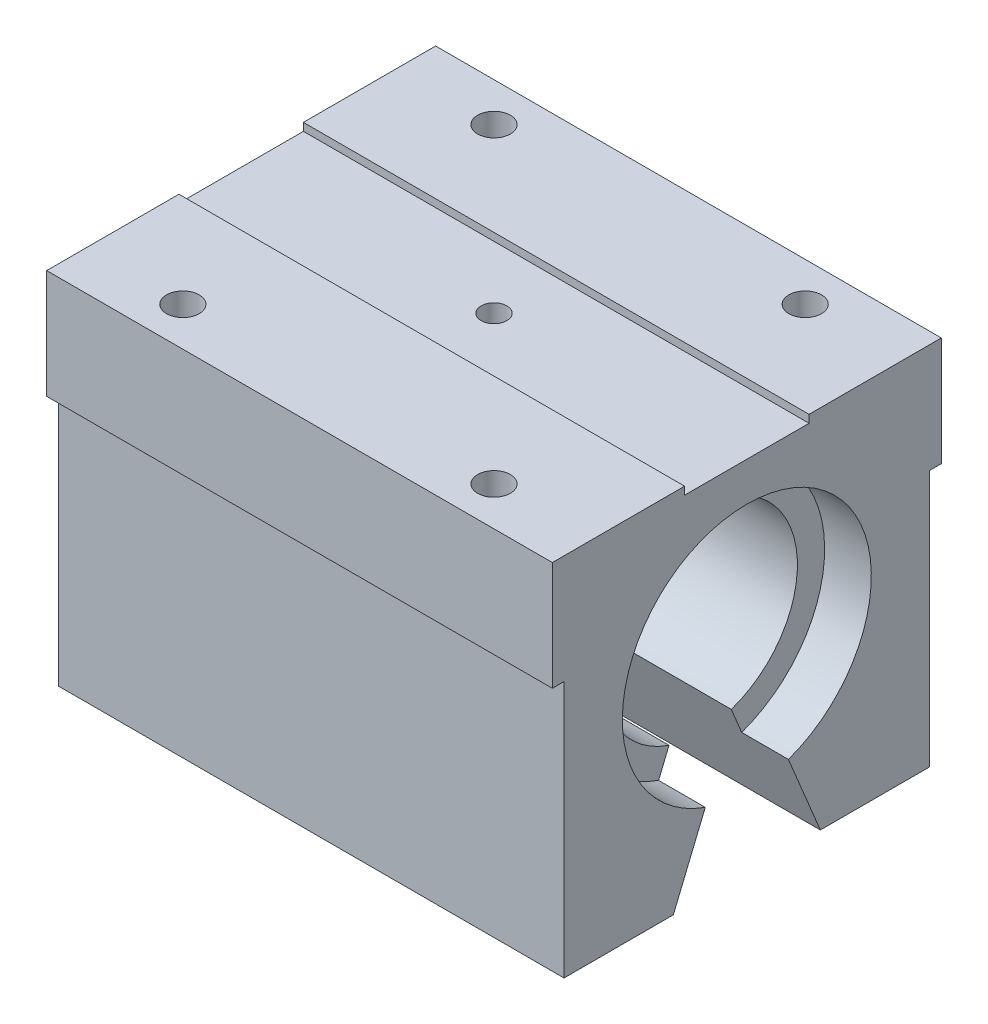
SolidWorks part; units mm, degrees
material "普通碳钢"
ref_plane "Front Plane" through (0, 0, 0) normal (0, 0, 1) x (1, 0, 0)
ref_plane "Top Plane" through (0, 0, 0) normal (0, 1, 0) x (1, 0, 0)
ref_plane "Right Plane" through (0, 0, 0) normal (1, 0, 0) x (0, 0, -1)
sketch "Sketch1" plane through (0, 0, 0) normal (1, 0, 0) x (0, 0, -1)
  line L0 (0, 0) -> (0, 31.1806) construction
  line L4 (-23.5, -25) -> (-9.4499, -25)
  line L5 (-25, 8) -> (-25, 22)
  line L6 (-8, 22) -> (-8, 21)
  line L8 (-8, 21) -> (8, 21)
  line L9 (-25, 22) -> (-8, 22)
  line L10 (8, 22) -> (8, 21)
  line L11 (8, 22) -> (25, 22)
  line L12 (-23.5, -25) -> (-23.5, 8)
  line L13 (23.5, -25) -> (23.5, 8)
  line L14 (-25, 8) -> (-23.5, 8)
  line L15 (25, 8) -> (25, 22)
  line L16 (-9.4499, -25) -> (-4, -11.8427)
  line L17 (23.5, 8) -> (25, 8)
  line L18 (9.4499, -25) -> (23.5, -25)
  line L20 (9.4499, -25) -> (4, -11.8427)
  arc A0 (4, -11.8427) -> (-4, -11.8427) centre (0, 0) ccw
  dimension "D1" = 25
  dimension "D7" = 22
  dimension "D10" = 8
  dimension "D2" = 45
  dimension "D3" = 47
  dimension "D4" = 50
  dimension "D5" = 16
  dimension "D6" = 1
  dimension "D8" = 1.5
  dimension "D9" = 14
extrude "Extrude1" add sketch "Sketch1" along normal blind 65
sketch "Sketch2" plane through (65, 0, 0) normal (1, 0, 0) x (0, 0, -1)
  circle A0 centre (0, 0) radius 16
  dimension "D1" = 32
extrude "Extrude2" cut sketch "Sketch2" against normal blind 6
sketch "Sketch3" plane through (0, 0, 0) normal (-1, 0, 0) x (0, 0, 1)
  arc A0 (5.3417, -15.082) -> (-5.3417, -15.082) centre (0, 0) ccw construction
  circle A2 centre (0, 0) radius 16
extrude "Extrude3" cut sketch "Sketch3" against normal blind 6
sketch "Sketch4" plane through (0, 22, 0) normal (0, 1, 0) x (1, 0, 0)
  line L0 (32.5, 25) -> (32.5, 0) construction
  line L1 (65, 25) -> (0, 25) construction
  line L2 (0, 0) -> (55.8292, 0) construction
  line L3 (12.5, -20) -> (52.5, -20) construction
  line L4 (12.5, -20) -> (12.5, 20) construction
  line L5 (12.5, 20) -> (52.5, 20) construction
  line L6 (52.5, -20) -> (52.5, 20) construction
  dimension "D1" = 40
  dimension "D2" = 40
hole_wizard "M5x0.8 Tapped Hole1" positions "3DSketch1" profile "Sketch5" tap size "M5x0.8" standard "Ansi Metric"
sketch3d "3DSketch1"
  point P0 (12.5, 22, -20)
  point P3 (52.5, 22, -20)
  point P6 (12.5, 22, 20)
  point P9 (52.5, 22, 20)
sketch "Sketch5" plane through (12.5, 22, -20) normal (1, 0, 0) x (0, 0, 1)
  line L0 (0, 0) -> (0, 13.6618)
  line L1 (0, 13.6618) -> (2.1, 12.4)
  line L2 (2.1, 12.4) -> (2.1, 0)
  line L5 (2.1, 0) -> (0, 0)
  line L10 (0, 13.6618) -> (-2.1, 12.4) construction
  line L11 (0, -6.35) -> (0, 107.95) construction
  dimension "螺纹孔钻头直径" = 4.2
  dimension "螺纹孔钻头深度" = 12.4
  dimension "导头角度" = 118
cosmetic thread "Hole Thread1" parameters "D1"=10, "D2"=5
cosmetic thread "Hole Thread2" parameters "D1"=10, "D2"=5
cosmetic thread "Hole Thread3" parameters "D1"=10, "D2"=5
cosmetic thread "Hole Thread4" parameters "D1"=10, "D2"=5
hole_wizard "M4x0.7 Tapped Hole1" positions "3DSketch2" profile "Sketch6" tap size "M4x0.7" standard "Ansi Metric"
sketch3d "3DSketch2"
  point P0 (32.5, 22, 0)
sketch "Sketch6" plane through (32.5, 22, 0) normal (1, 0, 0) x (0, 0, 1)
  line L0 (0, 0) -> (0, 11.0914)
  line L1 (0, 11.0914) -> (1.65, 10.1)
  line L2 (1.65, 10.1) -> (1.65, 0)
  line L5 (1.65, 0) -> (0, 0)
  line L10 (0, 11.0914) -> (-1.65, 10.1) construction
  line L11 (0, -6.35) -> (0, 107.95) construction
  dimension "螺纹孔钻头直径" = 3.3
  dimension "螺纹孔钻头深度" = 10.1
  dimension "导头角度" = 118
cosmetic thread "Hole Thread5" parameters "D1"=8, "D2"=4
